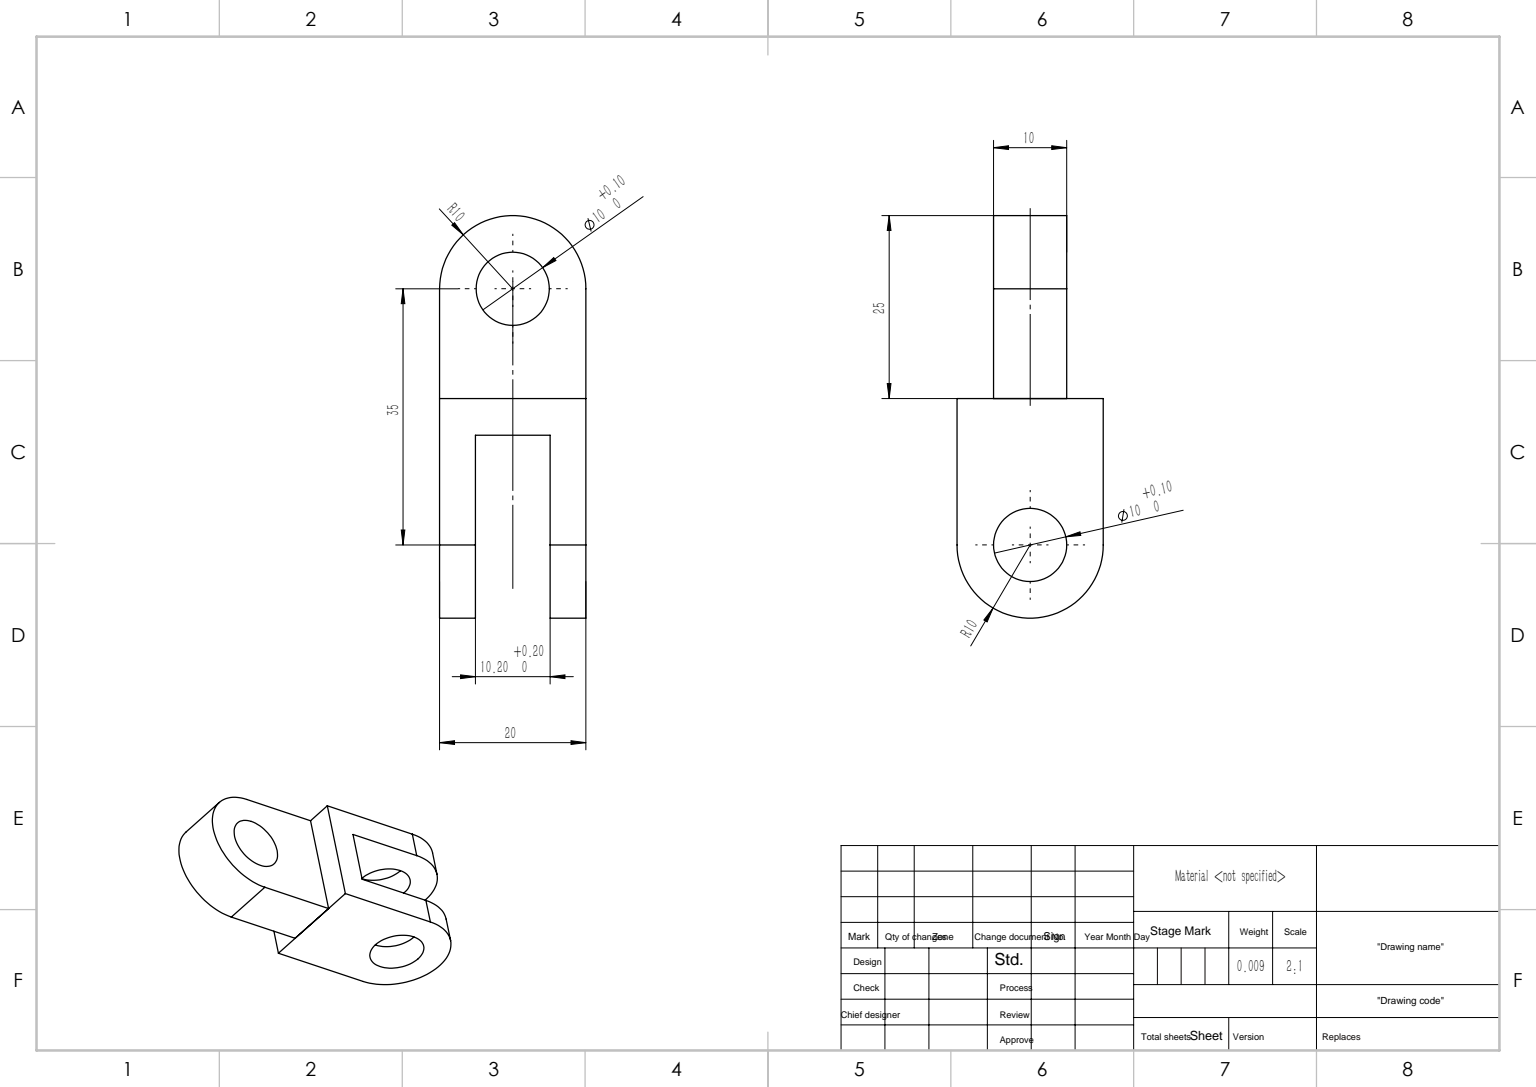
SolidWorks part; units mm, degrees
ref_plane "Front Plane" through (0, 0, 0) normal (0, 0, 1) x (1, 0, 0)
ref_plane "Top Plane" through (0, 0, 0) normal (0, 1, 0) x (1, 0, 0)
ref_plane "Right Plane" through (0, 0, 0) normal (1, 0, 0) x (0, 0, -1)
sketch "Sketch1" plane through (0, 0, 0) normal (0, 0, 1) x (1, 0, 0)
  line L0 (-10, 0) -> (-10, -15)
  line L1 (-10, -15) -> (10, -15)
  line L2 (10, -15) -> (10, 0)
  circle A0 centre (0, 0) radius 5
  arc A1 (10, 0) -> (-10, 0) centre (0, 0) ccw
  dimension "D1" = 10
  dimension "D2" = 20
  dimension "D3" = 15
extrude "Boss-Extrude1" add sketch "Sketch1" along normal blind 10
sketch "Sketch2" plane through (-10, 0, 0) normal (-1, 0, 0) x (0, 0, 1)
  line L0 (10, -15) -> (0, -15) construction
  line L1 (0, 0) -> (0, -15) construction
  line L2 (15, -35) -> (15, -15)
  line L3 (15, -15) -> (-5, -15)
  line L4 (-5, -15) -> (-5, -35)
  circle A0 centre (5, -35) radius 5
  arc A1 (-5, -35) -> (15, -35) centre (5, -35) ccw
  dimension "D1" = 20
  dimension "D2" = 20
  dimension "D3" = 10
  dimension "D4" = 5
extrude "Boss-Extrude2" add sketch "Sketch2" against normal blind 20 separate body
sketch "Sketch3" plane through (0, 0, -5) normal (0, 0, -1) x (-1, 0, 0)
  line L0 (-10, -15) -> (10, -15) construction
  line L1 (5.1, -20) -> (-5.1, -20)
  line L2 (5.1, -20) -> (5.1, -49.458)
  line L3 (5.1, -49.458) -> (-5.1, -49.458)
  line L4 (-5.1, -20) -> (-5.1, -49.458)
  line L5 (10, -15) -> (10, -35) construction
  line L6 (-10, -15) -> (-10, -35) construction
  dimension "D1" = 5
  dimension "D2" = 4.9
  dimension "D3" = 4.9
extrude "Cut-Extrude1" cut sketch "Sketch3" against normal through all
